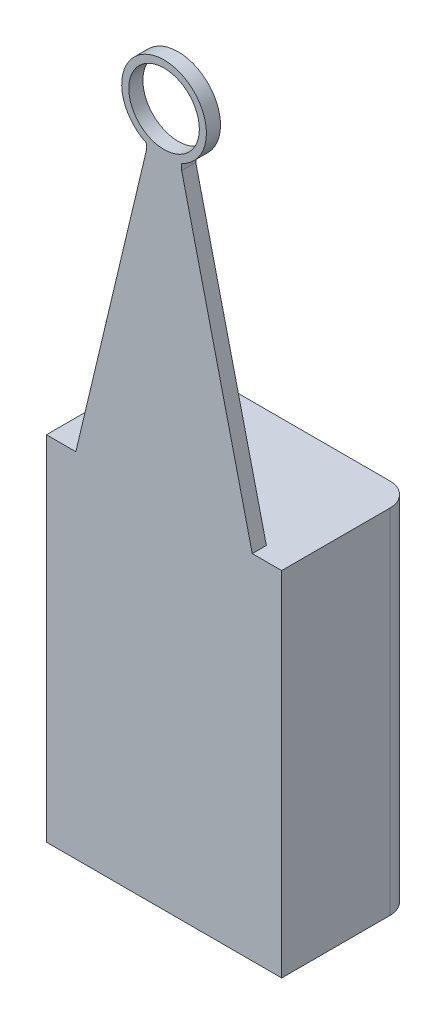
SolidWorks part; units mm, degrees
ref_plane "Front Plane" through (0, 0, 0) normal (0, 0, 1) x (1, 0, 0)
ref_plane "Top Plane" through (0, 0, 0) normal (0, 1, 0) x (1, 0, 0)
ref_plane "Right Plane" through (0, 0, 0) normal (1, 0, 0) x (0, 0, -1)
other "Configuration Table"
sketch "Sketch1" plane through (0, 0, 0) normal (0, 1, 0) x (1, 0, 0)
  line L1 (-10, 5.6) -> (10, 5.6)
  line L2 (-10, 5.6) -> (-10, -5.6)
  line L3 (-10, -5.6) -> (10, -5.6)
  line L4 (10, 5.6) -> (10, -5.6)
  line L5 (0, -5.6) -> (0, 5.6) construction
  line L6 (-10, 0) -> (10, 0) construction
  point P0 (0, 0)
  dimension "D1" = 11.2
  dimension "D2" = 20
extrude "Boss-Extrude1" add sketch "Sketch1" along normal blind 30
sketch "Sketch2" plane through (0, 0, 5.6) normal (0, 0, 1) x (1, 0, 0)
  line L0 (-10, 0) -> (10, 0) construction
  line L1 (0, 59) -> (0, 0) construction
  line L2 (-1.5, 55.1974) -> (-7.5, 30)
  line L3 (-1.5, 55.7274) -> (-1.5, 55.1974)
  line L5 (-10, 30) -> (10, 30) construction
  line L6 (1.5, 55.7274) -> (1.5, 55.1974)
  line L7 (1.5, 55.1974) -> (7.5, 30)
  line L8 (7.5, 30) -> (-7.5, 30)
  circle A0 centre (0, 59) radius 3
  arc A1 (1.5, 55.7274) -> (-1.5, 55.7274) centre (0, 59) ccw
  dimension "D1" = 6
  dimension "D3" = 7.2
  dimension "D2" = 59
  dimension "D4" = 3
  dimension "D5" = 0.53
  dimension "D6" = 15
extrude "Boss-Extrude2" add sketch "Sketch2" against normal blind 1.2
fillet "Fillet1" radius 2 2 edges at (-10, 15, -5.6) (10, 15, -5.6)
ref_plane "Plane1" through (0, 0, 8.6) normal (0, 0, 1) x (1, 0, 0)
sketch "Sketch3" plane through (0, 0, 0) normal (0, -1, 0) x (1, 0, 0)
  line L0 (0, 0) -> (0, -5.6) construction
  line L1 (8, -5.6) -> (-8, -5.6) construction
  line L2 (6.5, -5.6) -> (4, -5.6)
  line L3 (-6.5, -5.6) -> (-4, -5.6)
  line L4 (-6.5, -5.6) -> (-6.5, -6.85)
  line L6 (-4, -5.6) -> (-4, -6.85)
  line L7 (4, -5.6) -> (4, -6.85)
  line L8 (6.5, -5.6) -> (6.5, -6.85)
  arc A0 (-6.5, -6.85) -> (-4, -6.85) centre (-5.25, -6.85) ccw
  circle A1 centre (-5.25, -6.85) radius 0.6
  circle A2 centre (5.25, -6.85) radius 0.6
  arc A3 (6.5, -6.85) -> (4, -6.85) centre (5.25, -6.85) cw
  point P9 (-6.5, -6.225)
  dimension "D4" = 2.5
  dimension "D1" = 1.2
  dimension "D2" = 2.5
  dimension "D3" = 4
extrude "Boss-Extrude3" add sketch "Sketch3" against normal blind 1
